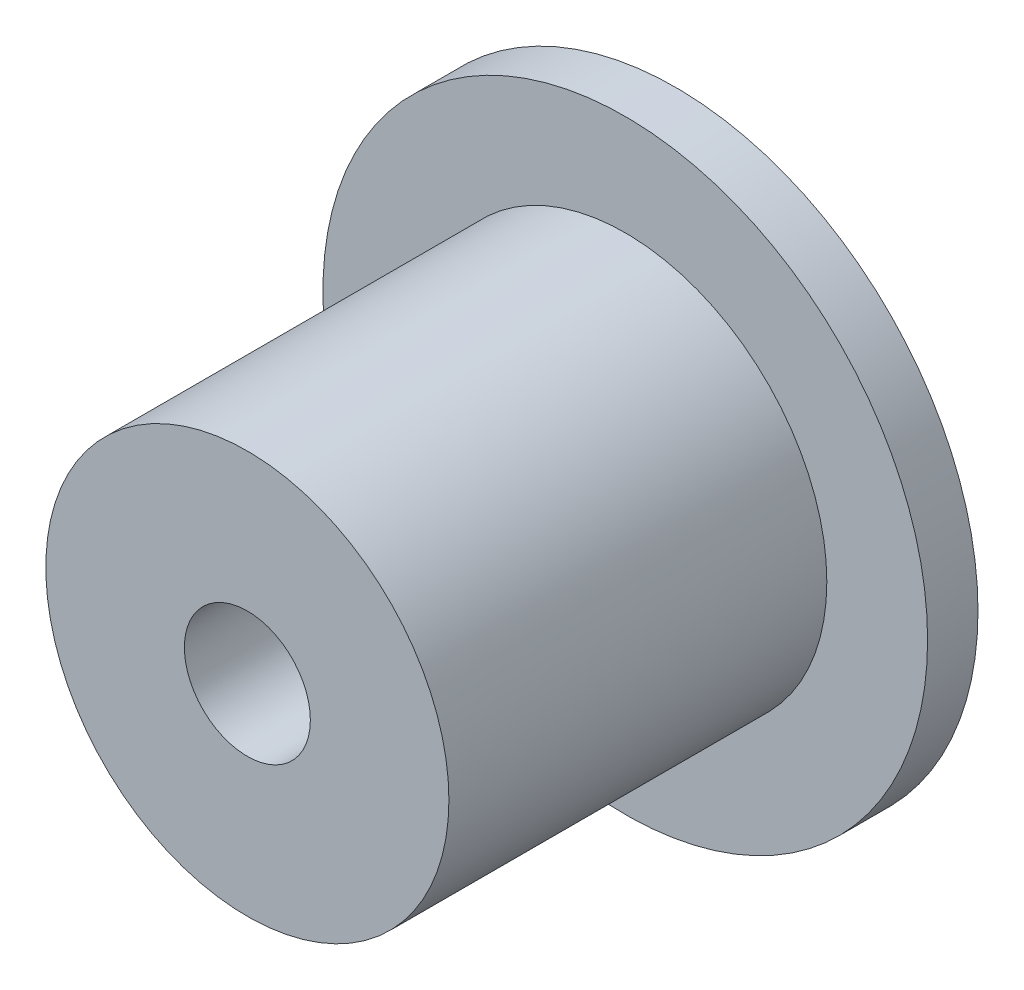
from build123d import *

# Parameters (mm, degrees)
SKETCH_1_R      = 4
SKETCH_1_R_2    = 1.25
EXTRUDE_1_DEPTH = 7.5
EXTRUDE_START   = -1
SKETCH_2_R      = 6
SKETCH_2_R_2    = 1.25
EXTRUDE_2_DEPTH = 1


with BuildPart() as part:
    # 草图1 → 凸台-拉伸1 (new body)
    with BuildSketch(Plane.XY):
        Circle(SKETCH_1_R)
        Circle(SKETCH_1_R_2, mode=Mode.SUBTRACT)
    extrude(amount=EXTRUDE_1_DEPTH)

    # 草图2 → 凸台-拉伸2 (add)
    with BuildSketch(Plane.XY.offset(EXTRUDE_START)):
        Circle(SKETCH_2_R)
        Circle(SKETCH_2_R_2, mode=Mode.SUBTRACT)
    extrude(amount=EXTRUDE_2_DEPTH)


solid = part.part
